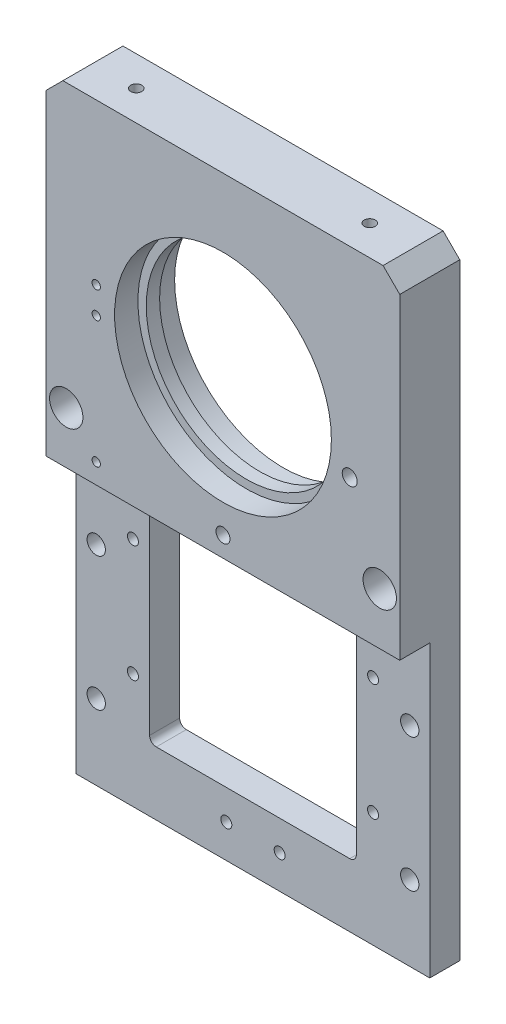
SolidWorks part; units mm, degrees
ref_plane "Front Plane" through (0, 0, 0) normal (0, 0, 1) x (1, 0, 0)
ref_plane "Top Plane" through (0, 0, 0) normal (0, 1, 0) x (1, 0, 0)
ref_plane "Right Plane" through (0, 0, 0) normal (1, 0, 0) x (0, 0, -1)
sketch "Sketch1" plane through (0, 0, 0) normal (0, 0, 1) x (1, 0, 0)
  line L1 (-53, 93.5) -> (53, 93.5)
  line L2 (-53, 93.5) -> (-53, -93.5)
  line L3 (-53, -93.5) -> (53, -93.5)
  line L4 (53, 93.5) -> (53, -93.5)
  line L5 (-53, 93.5) -> (53, -93.5) construction
  line L6 (-53, -93.5) -> (53, 93.5) construction
  point P0 (0, 0)
  dimension "D1" = 106
  dimension "D2" = 187
extrude "Boss-Extrude1" add sketch "Sketch1" along normal mid plane 18
sketch "Sketch2" plane through (0, 0, -9) normal (0, 0, -1) x (-1, 0, 0)
  line L1 (-53, 93.5) -> (53, 93.5) construction
  circle A0 centre (0, 40.5) radius 30
  dimension "D1" = 60
  dimension "D2" = 53
extrude "Cut-Extrude1" cut sketch "Sketch2" against normal through all
sketch "Sketch3" plane through (0, 0, 9) normal (0, 0, 1) x (1, 0, 0)
  circle A0 centre (0, 40.5) radius 32.5
  dimension "D1" = 65
extrude "Cut-Extrude2" cut sketch "Sketch3" against normal blind 7
sketch "Sketch4" plane through (0, 0, -9) normal (0, 0, -1) x (-1, 0, 0)
  circle A0 centre (0, 40.5) radius 32.5
  dimension "D1" = 65
extrude "Cut-Extrude3" cut sketch "Sketch4" against normal blind 7
sketch "Sketch5" plane through (0, 0, 9) normal (0, 0, 1) x (1, 0, 0)
  line L0 (0, 0) -> (0, -56.2195) construction
  line L1 (-31, -74.5) -> (31, -74.5)
  line L2 (-31, -74.5) -> (-31, -6.5)
  line L3 (-31, -6.5) -> (31, -6.5)
  line L4 (31, -74.5) -> (31, -6.5)
  line L6 (53, 93.5) -> (-53, 93.5) construction
  dimension "D1" = 62
  dimension "D2" = 68
  dimension "D3" = 100
extrude "Cut-Extrude4" cut sketch "Sketch5" against normal through all
fillet "Fillet1" radius 2 4 edges at (-31, -74.5, 0) (31, -74.5, 0) (31, -6.5, 0) (-31, -6.5, 0)
sketch "Sketch6" plane through (53, 0, 0) normal (1, 0, 0) x (0, 0, -1)
  line L0 (9, -93.5) -> (9, 93.5) construction
  line L1 (-9, -93.5) -> (0, -93.5)
  line L2 (-9, -93.5) -> (-9, -6.5)
  line L3 (-9, -6.5) -> (0, -6.5)
  line L4 (0, -93.5) -> (0, -6.5)
  line L5 (-9, 93.5) -> (9, 93.5) construction
  dimension "D1" = 9
  dimension "D2" = 100
extrude "Cut-Extrude5" cut sketch "Sketch6" against normal through all
hole_wizard "M4 Tapped Hole1" positions "Sketch8" profile "Sketch7" tap size "M4" standard "Gb" end condition through all
sketch "Sketch8" plane through (0, 0, 0) normal (0, 0, 1) x (1, 0, 0)
  line L1 (0, 0) -> (0, -60) construction
  line L2 (53, 93.5) -> (-53, 93.5) construction
  point P0 (36, -24)
  point P2 (36, -59)
  point P4 (-36, -59)
  point P6 (-36, -24)
  dimension "D1" = 35
  dimension "D2" = 117.5
  dimension "D3" = 72
sketch "Sketch7" plane through (36, -24, 0) normal (1, 0, 0) x (0, -1, 0)
  line L0 (0, 0) -> (0, 9)
  line L1 (0, 9) -> (1.65, 9)
  line L2 (1.65, 9) -> (1.65, 0)
  line L5 (1.65, 0) -> (0, 0)
  line L11 (0, -6.35) -> (0, 107.95) construction
  dimension "通孔螺纹孔钻头直径" = 3.3
  dimension "通孔螺纹孔钻头深度" = 9
cosmetic thread "Hole Thread1" parameters "D2"=4
cosmetic thread "Hole Thread2" parameters "D2"=4
cosmetic thread "Hole Thread3" parameters "D2"=4
cosmetic thread "Hole Thread4" parameters "D2"=4
hole_wizard "M4 Tapped Hole2" positions "Sketch10" profile "Sketch9" tap size "M4" standard "Gb" end condition through all
sketch "Sketch10" plane through (0, 0, 0) normal (0, 0, 1) x (1, 0, 0)
  line L0 (-53, -93.5) -> (53, -93.5) construction
  line L1 (0, 0) -> (0, -88.1197) construction
  point P0 (-8, -83.5)
  point P3 (8, -83.5)
  dimension "D1" = 16
  dimension "D2" = 10
sketch "Sketch9" plane through (-8, -83.5, 0) normal (1, 0, 0) x (0, -1, 0)
  line L0 (0, 0) -> (0, 9)
  line L1 (0, 9) -> (1.65, 9)
  line L2 (1.65, 9) -> (1.65, 0)
  line L5 (1.65, 0) -> (0, 0)
  line L11 (0, -6.35) -> (0, 107.95) construction
  dimension "通孔螺纹孔钻头直径" = 3.3
  dimension "通孔螺纹孔钻头深度" = 9
cosmetic thread "Hole Thread5" parameters "D2"=4
cosmetic thread "Hole Thread6" parameters "D2"=4
hole_wizard "M3 Tapped Hole1" positions "Sketch12" profile "Sketch11" tap size "M3" standard "Gb"
sketch "Sketch12" plane through (0, 0, 9) normal (0, 0, 1) x (1, 0, 0)
  line L2 (-53, 93.5) -> (-53, -6.5) construction
  line L3 (53, 93.5) -> (-53, 93.5) construction
  line L4 (53, -6.5) -> (-53, -6.5) construction
  point P0 (-38, 45.5)
  point P3 (-38, 37.5)
  point P26 (-38, -0.5)
  dimension "D1" = 8
  dimension "D2" = 15
  dimension "D3" = 48
  dimension "D4" = 6
sketch "Sketch11" plane through (-38, 45.5, 9) normal (1, 0, 0) x (0, -1, 0)
  line L0 (0, 0) -> (0, 8.2511)
  line L1 (0, 8.2511) -> (1.25, 7.5)
  line L2 (1.25, 7.5) -> (1.25, 0)
  line L5 (1.25, 0) -> (0, 0)
  line L10 (0, 8.2511) -> (-1.25, 7.5) construction
  line L11 (0, -6.35) -> (0, 107.95) construction
  dimension "螺纹孔钻头直径" = 2.5
  dimension "螺纹孔钻头深度" = 7.5
  dimension "导头角度" = 118
cosmetic thread "Hole Thread7" parameters "D1"=6, "D2"=3
cosmetic thread "Hole Thread8" parameters "D1"=6, "D2"=3
cosmetic thread "Hole Thread12" parameters "D1"=6, "D2"=3
chamfer "Chamfer1" distance 5 angle 45 2 edges at (53, 93.5, 0) (-53, 93.5, 0)
hole_wizard "Hole size per socket head cap screw type1" positions "Sketch14" profile "Sketch13" counterbore size "M4" standard "Gb" end condition through all
sketch "Sketch14" plane through (0, 0, -9) normal (0, 0, -1) x (-1, 0, 0)
  line L0 (-53, -93.5) -> (-53, 88.5) construction
  line L1 (-48, 93.5) -> (48, 93.5) construction
  point P0 (-38, 33.5)
  dimension "D1" = 15
  dimension "D2" = 60
sketch "Sketch13" plane through (38, 33.5, -9) normal (1, 0, 0) x (0, 1, 0)
  line L0 (0, 0) -> (0, 18)
  line L1 (0, 18) -> (2.25, 18)
  line L3 (2.25, 18) -> (2.25, 5)
  line L4 (2.25, 5) -> (4, 5)
  line L5 (4, 5) -> (4, 0)
  line L7 (4, 0) -> (0, 0)
  line L11 (0, -6.35) -> (0, 107.95) construction
  dimension "通孔孔直径" = 4.5
  dimension "通孔孔深度" = 18
  dimension "柱形沉头孔直径" = 8
  dimension "柱形沉头孔深度" = 5
hole_wizard "Hole size per socket head cap screw type2" positions "Sketch16" profile "Sketch15" counterbore size "M5" standard "Gb" end condition through all
sketch "Sketch16" plane through (0, 0, 9) normal (0, 0, 1) x (1, 0, 0)
  line L0 (0, 0) -> (0, -101.3375) construction
  line L2 (-53, -93.5) -> (53, -93.5) construction
  point P0 (-47, 9.0574)
  point P3 (-47, -30.9426)
  point P6 (-47, -70.9426)
  point P9 (47, -70.9426)
  point P12 (47, -30.9426)
  point P15 (47, 9.0574)
  dimension "D1" = 94
  dimension "D2" = 22.5574
  dimension "D3" = 40
  dimension "D4" = 40
sketch "Sketch15" plane through (-47, 9.0574, 9) normal (1, 0, 0) x (0, -1, 0)
  line L0 (0, 0) -> (0, 18)
  line L1 (0, 18) -> (2.75, 18)
  line L3 (2.75, 18) -> (2.75, 9)
  line L4 (2.75, 9) -> (5, 9)
  line L5 (5, 9) -> (5, 0)
  line L7 (5, 0) -> (0, 0)
  line L11 (0, -6.35) -> (0, 107.95) construction
  dimension "通孔孔直径" = 5.5
  dimension "通孔孔深度" = 18
  dimension "柱形沉头孔直径" = 10
  dimension "柱形沉头孔深度" = 9
hole_wizard "M5 Tapped Hole1" positions "Sketch18" profile "Sketch17" tap size "M5" standard "Gb"
sketch "Sketch18" plane through (0, 0, 9) normal (0, 0, 1) x (1, 0, 0)
  line L0 (53, -6.5) -> (-53, -6.5) construction
  point P0 (0, -0.5)
  dimension "D1" = 6
cosmetic thread "Hole Thread9" parameters "D1"=10, "D2"=5
sketch "Sketch17" plane through (0, -0.5, 9) normal (1, 0, 0) x (0, -1, 0)
  line L0 (0, 0) -> (0, 13.6618)
  line L1 (0, 13.6618) -> (2.1, 12.4)
  line L2 (2.1, 12.4) -> (2.1, 0)
  line L5 (2.1, 0) -> (0, 0)
  line L10 (0, 13.6618) -> (-2.1, 12.4) construction
  line L11 (0, -6.35) -> (0, 107.95) construction
  dimension "螺纹孔钻头直径" = 4.2
  dimension "螺纹孔钻头深度" = 12.4
  dimension "导头角度" = 118
hole_wizard "M4 Tapped Hole3" positions "Sketch20" profile "Sketch19" tap size "M4" standard "Gb"
sketch "Sketch20" plane through (0, 93.5, 0) normal (0, 1, 0) x (1, 0, 0)
  line L0 (0, 0) -> (0, 20.367) construction
  point P0 (-35, 0)
  point P2 (35, 0)
  dimension "D1" = 70
sketch "Sketch19" plane through (-35, 93.5, 0) normal (1, 0, 0) x (0, 0, 1)
  line L0 (0, 0) -> (0, 13.0914)
  line L1 (0, 13.0914) -> (1.65, 12.1)
  line L2 (1.65, 12.1) -> (1.65, 0)
  line L5 (1.65, 0) -> (0, 0)
  line L10 (0, 13.0914) -> (-1.65, 12.1) construction
  line L11 (0, -6.35) -> (0, 107.95) construction
  dimension "螺纹孔钻头直径" = 3.3
  dimension "螺纹孔钻头深度" = 12.1
  dimension "导头角度" = 118
cosmetic thread "Hole Thread10" parameters "D1"=10, "D2"=4
cosmetic thread "Hole Thread11" parameters "D1"=10, "D2"=4
